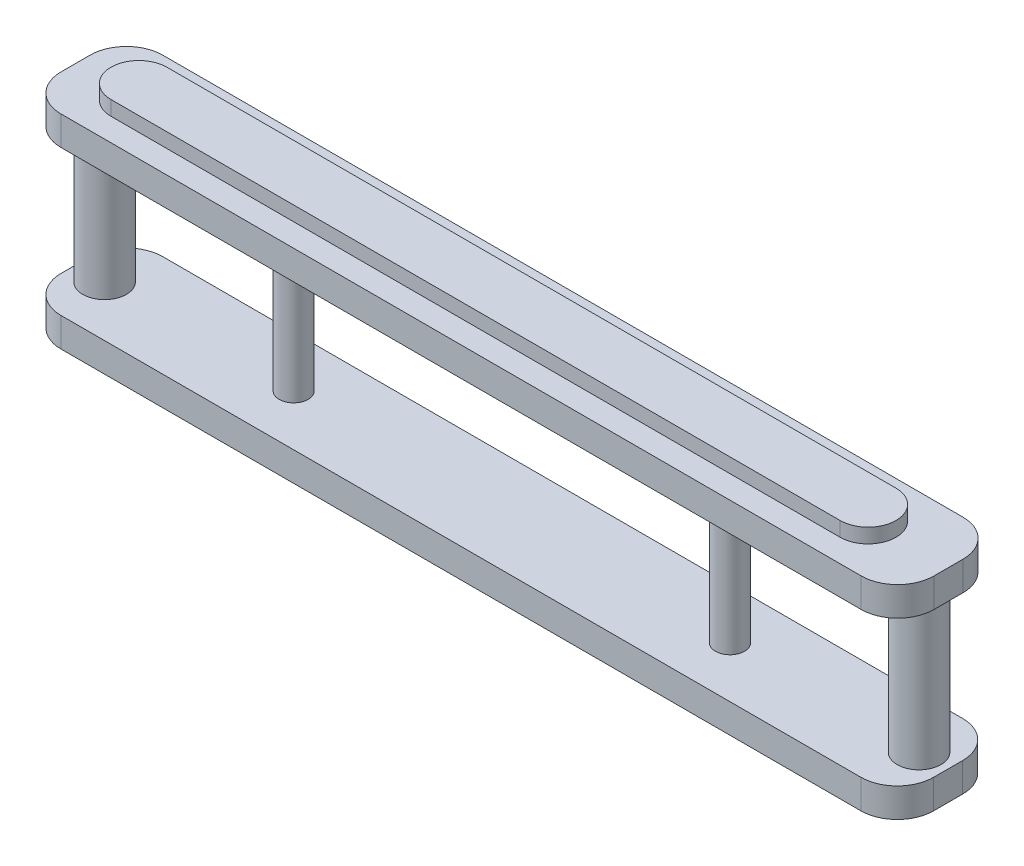
SolidWorks part; units mm, degrees
ref_plane "Front Plane" through (0, 0, 0) normal (0, 0, 1) x (1, 0, 0)
ref_plane "Top Plane" through (0, 0, 0) normal (0, 1, 0) x (1, 0, 0)
ref_plane "Right Plane" through (0, 0, 0) normal (1, 0, 0) x (0, 0, -1)
sketch "Sketch3" plane through (0, 0, 0) normal (0, 1, 0) x (1, 0, 0)
  line L1 (-3000, 350) -> (3000, 350)
  line L2 (-3000, 350) -> (-3000, -350)
  line L3 (-3000, -350) -> (3000, -350)
  line L4 (3000, 350) -> (3000, -350)
  line L5 (-3000, 350) -> (3000, -350) construction
  line L6 (-3000, -350) -> (3000, 350) construction
  point P0 (0, 0)
  dimension "D1" = 6000
  dimension "D2" = 700
extrude "Boss-Extrude3" add sketch "Sketch3" along normal blind 200
sketch "Sketch4" plane through (0, 200, 0) normal (0, 1, 0) x (1, 0, 0)
  line L0 (-2800, 0) -> (2800, 0) construction
  circle A0 centre (-2800, 0) radius 150
  circle A1 centre (2800, 0) radius 150
  circle A2 centre (-1500, 0) radius 100
  circle A3 centre (1500, 0) radius 100
  point P4 (0, 0)
  dimension "D2" = 300
  dimension "D3" = 300
  dimension "D4" = 200
  dimension "D5" = 200
  dimension "D1" = 5600
  dimension "D6" = 1300
  dimension "D7" = 1300
extrude "Boss-Extrude4" add sketch "Sketch4" along normal blind 1000
sketch "Sketch5" plane through (0, 1200, 0) normal (0, 1, 0) x (1, 0, 0)
  line L0 (-3000, 350) -> (-3000, -350)
  line L1 (-3000, 350) -> (3002.2194, 350)
  line L2 (-3000, -350) -> (3002.2194, -350)
  line L3 (3002.2194, 350) -> (3002.2194, -350)
extrude "Boss-Extrude5" add sketch "Sketch5" along normal blind 200
fillet "Fillet1" radius 250 8 edges at (3002.2194, 1300, -350) (3002.2194, 1300, 350) (3000, 100, -350) (3000, 100, 350) (-3000, 100, -350) (-3000, 1300, -350) (-3000, 1300, 350) (-3000, 100, 350)
sketch "Sketch6" plane through (0, 0, 0) normal (0, -1, 0) x (1, 0, 0)
  line L0 (-2564.073, 0) -> (2449.5371, 0) construction
  line L1 (-2564.073, 192.3029) -> (2449.5371, 192.3029)
  line L2 (-2564.073, -192.3029) -> (2449.5371, -192.3029)
  arc A0 (-2564.073, 192.3029) -> (-2564.073, -192.3029) centre (-2564.073, 0) ccw
  arc A1 (2449.5371, -192.3029) -> (2449.5371, 192.3029) centre (2449.5371, 0) ccw
  point P3 (-57.2679, 0)
extrude "Boss-Extrude6" add sketch "Sketch6" along normal blind 100
ref_plane "Plane1" through (0, 700, 0) normal (0, 1, 0) x (1, 0, 0)
mirror "Mirror1" about plane through (0, 700, 0) normal (0, 1, 0) of "Boss-Extrude6"
